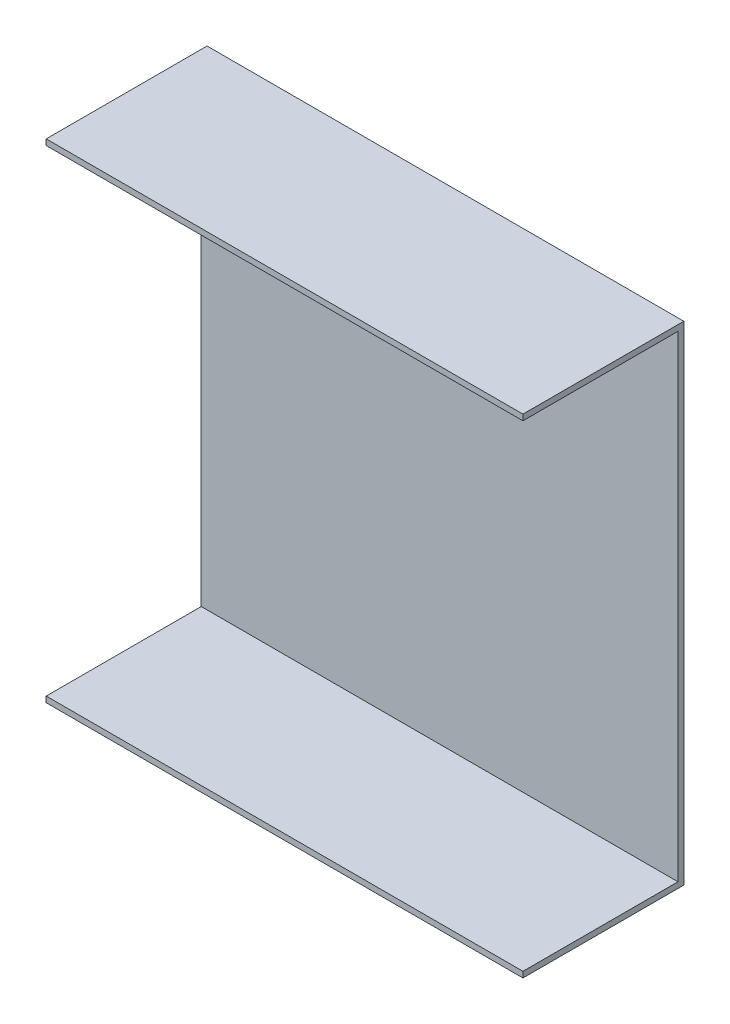
from build123d import *

# Parameters (mm, degrees)
SKETCH1_W           = 246
SKETCH1_H           = 252
BOSS_EXTRUDE1_DEPTH = 3
SKETCH2_W           = 246
SKETCH2_H           = 3
BOSS_EXTRUDE2_DEPTH = 80


with BuildPart() as part:
    # Sketch1 → Boss-Extrude1 (new body)
    with BuildSketch(Plane.XY):
        Rectangle(SKETCH1_W, SKETCH1_H)
    extrude(amount=BOSS_EXTRUDE1_DEPTH)

    # Sketch2 → Boss-Extrude2 (add)
    with BuildSketch(Plane.XY.offset(3)):
        with Locations((0, 124.5)):
            Rectangle(SKETCH2_W, SKETCH2_H)
        with Locations((0, -124.5)):
            Rectangle(SKETCH2_W, SKETCH2_H)
    extrude(amount=BOSS_EXTRUDE2_DEPTH)


solid = part.part
